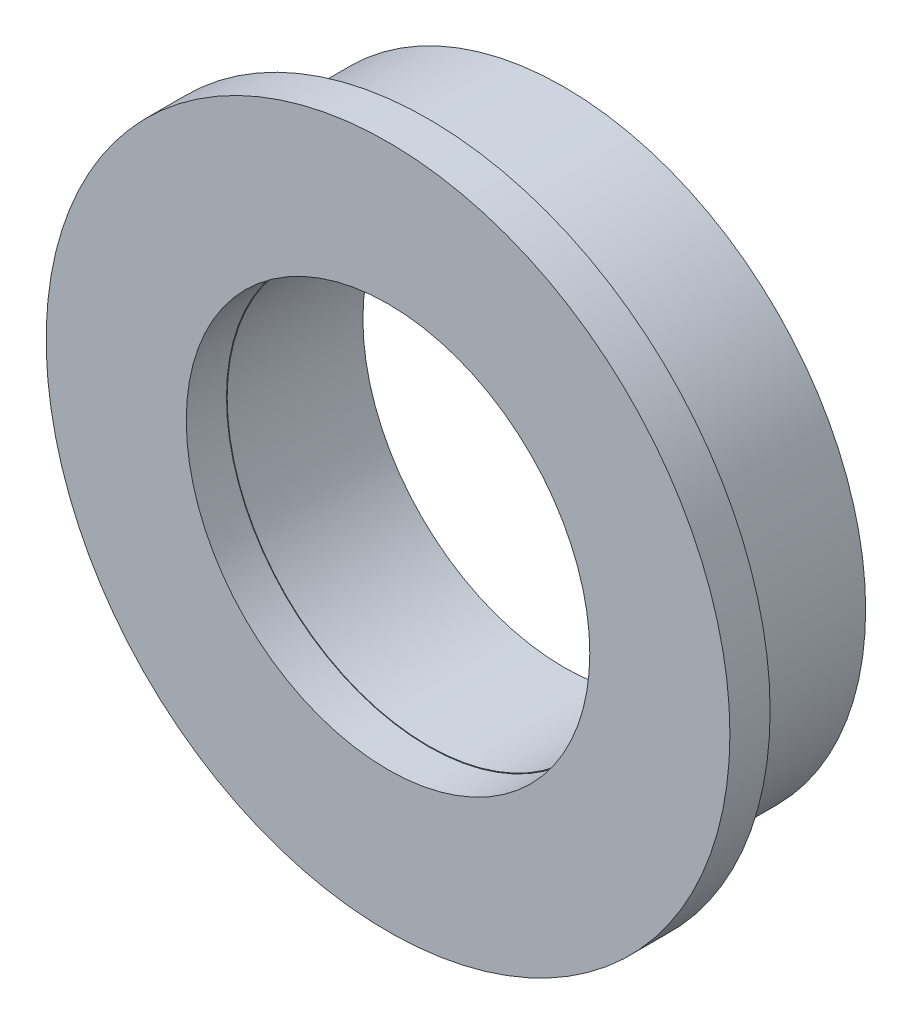
SolidWorks part; units mm, degrees
ref_plane "前视基准面" through (0, 0, 0) normal (0, 0, 1) x (1, 0, 0)
ref_plane "上视基准面" through (0, 0, 0) normal (0, 1, 0) x (1, 0, 0)
ref_plane "右视基准面" through (0, 0, 0) normal (1, 0, 0) x (0, 0, -1)
sketch "草图1" plane through (0, 0, 0) normal (0, 0, 1) x (1, 0, 0)
  circle A0 centre (0, 0) radius 4
  circle A1 centre (0, 0) radius 6
  dimension "D1" = 8
  dimension "D2" = 12
extrude "凸台-拉伸1" add sketch "草图1" along normal blind 2.7
sketch "草图2" plane through (0, 0, 2.7) normal (0, 0, 1) x (1, 0, 0)
  circle A0 centre (0, 0) radius 4.0134
  circle A1 centre (0, 0) radius 6.8
  dimension "D1" = 13.6
extrude "凸台-拉伸2" add sketch "草图2" along normal blind 0.8
